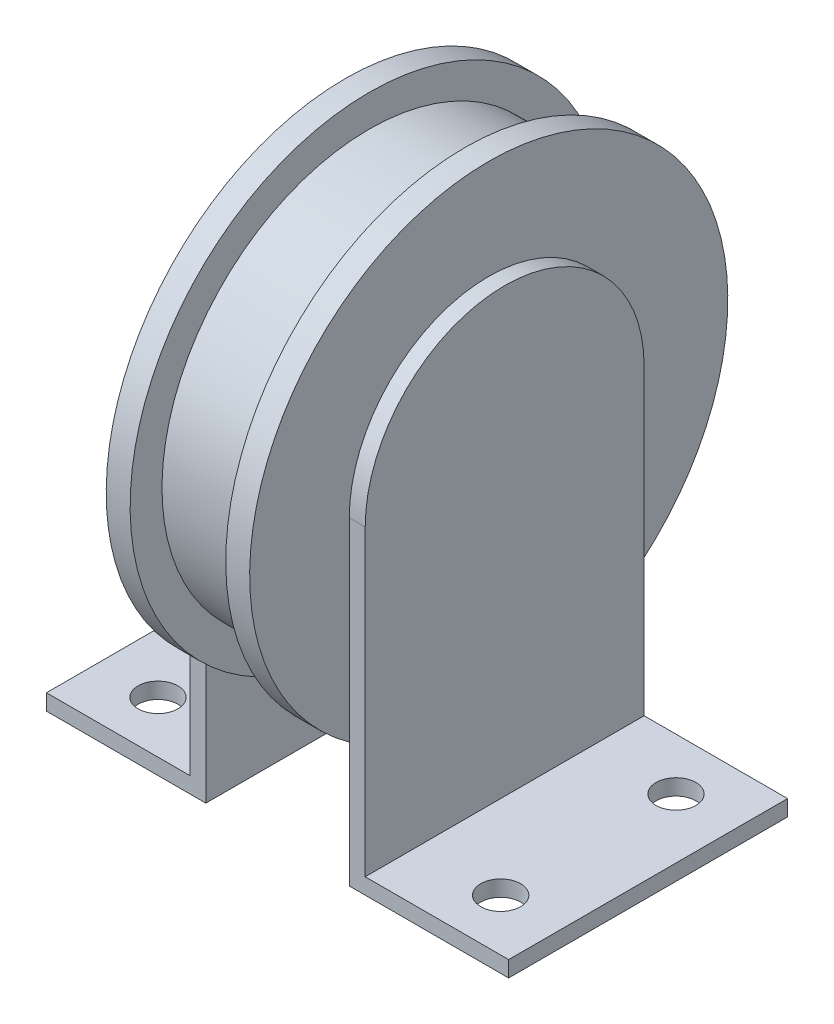
SolidWorks part; units mm, degrees
ref_plane "前视基准面" through (0, 0, 0) normal (0, 0, 1) x (1, 0, 0)
ref_plane "上视基准面" through (0, 0, 0) normal (0, 1, 0) x (1, 0, 0)
ref_plane "右视基准面" through (0, 0, 0) normal (1, 0, 0) x (0, 0, -1)
sketch "草图1" plane through (0, 0, 0) normal (0, 0, 1) x (1, 0, 0)
  line L0 (0, 18.5506) -> (0, -27.6705) construction
  line L1 (0, 30) -> (3, 30)
  line L2 (3, 30) -> (3, 26)
  line L3 (3, 26) -> (15, 26)
  line L4 (15, 26) -> (15, 30)
  line L5 (15, 30) -> (18, 30)
  line L6 (18, 30) -> (18, 0)
  line L7 (18, 0) -> (-18, 0)
  line L8 (0, 30) -> (0, 0)
  point P12 (0, 0)
  dimension "D1" = 12
  dimension "D2" = 30
  dimension "D3" = 3
  dimension "D4" = 3
  dimension "D5" = 26
revolve "旋转1" add sketch "草图1" angle 360 about L7
ref_plane "基准面1" through (9, 0, 0) normal (1, 0, 0) x (0, 0, -1)
sketch "草图2" plane through (18, 0, 0) normal (1, 0, 0) x (0, 0, -1)
  line L0 (-17.5, 0) -> (-17.5, -40)
  line L1 (-17.5, -40) -> (17.5, -40)
  line L2 (17.5, -40) -> (17.5, 0)
  circle A0 centre (0, 0) radius 17.5
  circle M2 centre (0, 0) radius 30
  dimension "D1" = 35
  dimension "D2" = 40
extrude "凸台-拉伸1" add sketch "草图2" along normal blind 2 contours A0 | A0 L0 L2 M2 | L1 L2 L0 M2
sketch "草图3" plane through (20, 0, 0) normal (1, 0, 0) x (0, 0, -1)
  line L0 (17.5, -40) -> (17.5, 0) construction
  line L1 (-17.5, -40) -> (17.5, -40)
  line L2 (-17.5, -40) -> (-17.5, -38)
  line L3 (-17.5, -38) -> (17.5, -38)
  line L4 (17.5, -40) -> (17.5, -38)
  dimension "D1" = 2
extrude "凸台-拉伸2" add sketch "草图3" along normal blind 18
mirror "镜向1" about plane through (9, 0, 0) normal (1, 0, 0) of "凸台-拉伸2", "凸台-拉伸1"
sketch "草图4" plane through (0, -40, 0) normal (0, -1, 0) x (1, 0, 0)
  line L0 (9, 33.4993) -> (9, -34.5699) construction
  line L1 (9, -33) -> (9, 33) construction
  line L2 (-20, 0) -> (49.3241, 0) construction
  line L3 (-20, 17.5) -> (-20, -17.5) construction
  circle A0 centre (-12.5, 11) radius 2.5
  circle A1 centre (-12.5, -11) radius 2.5
  circle A2 centre (30.5, -11) radius 2.5
  circle A3 centre (30.5, 11) radius 2.5
  dimension "D1" = 5
  dimension "D2" = 43
  dimension "D3" = 22
extrude "切除-拉伸1" cut sketch "草图4" against normal up to next
